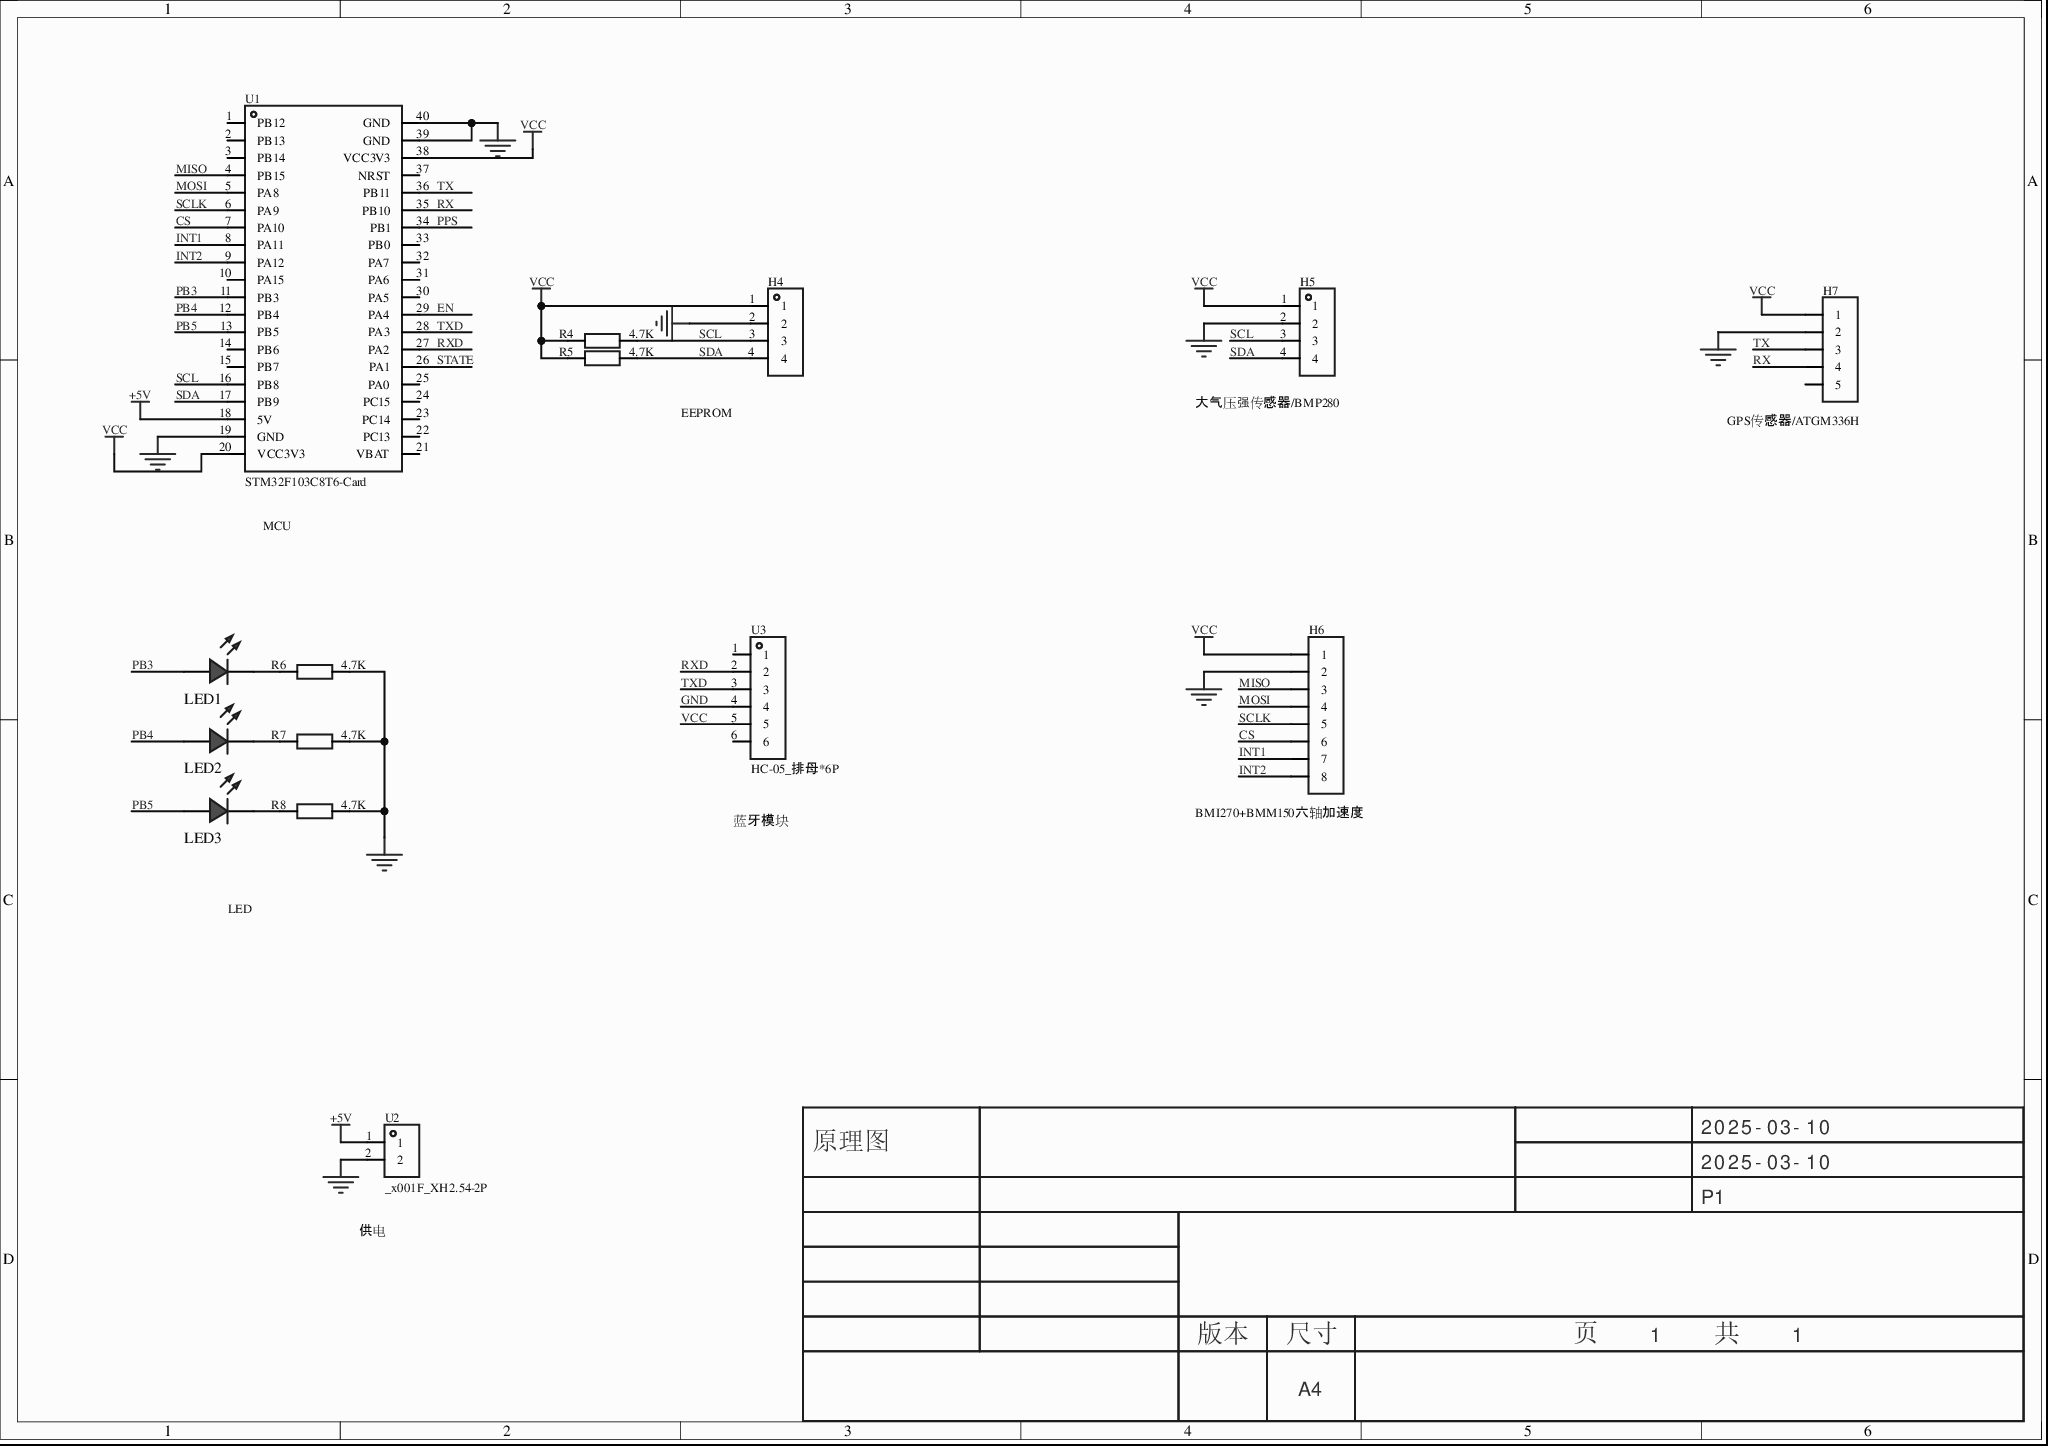
[diagram p0: MISC51830-3.schdoc]
# Altium project MISC51830-2.PrjPcb
1 sheet, 15 parts. Net scope: global (net labels, ports and power ports of the same name join across sheets).
Board file: MISC51830.pcbdoc

## Sheet MISC51830-3.schdoc
size 297 x 209 mm; Version: V1.0; @Project Name: MISC51830; @Page Count: 1; @Update Date: 2025-03-10; @Create Date: 2025-03-10; @Schematic Name: MISC51830; @Page No: 1; @Create Time: 12:29:11; @Update Time: 12:29:16; @Board Name: MISC51830

### Parts
H4  (no value)  [HDR-TH_4P-P2.54-V-F]
H5  (no value)  [HDR-TH_4P-P2.54-V-F]
H6  (no value)  [HDR-TH_8P-P2.54-V-F-1]
H7  (no value)  [HDR-TH_5P-P2.54-V-F]
LED1  (no value)  [LED_0805]
LED2  (no value)  [LED_0805]
LED3  (no value)  [LED_0805]
R4  4.7K  [R0805]
R5  4.7K  [R0805]
R6  4.7K  [R0805]
R7  4.7K  [R0805]
R8  4.7K  [R0805]
U1  STM32F103C8T6-Card  [CONN-TH_L53.3-W22.9_STM32F103C8T6-CARD]
U2  _x001F_XH2.54-2P  [CONN-TH_2P-P2.54-V]
U3  HC-05_排母*6P  [HDR-TH_6P-P2.50-V-F-R1-C6]

### Nets
+5V: U1.18(5V) U2.1
GND: H4.2 H5.2 H6.2 H7.2 R6.2 R7.2 R8.2 U1.19(GND) U1.39(GND) U1.40(GND) U2.2 U3.4
VCC: H4.1 H5.1 H6.1 H7.1 R4.1 R5.1 U1.20(VCC3V3) U1.38(VCC3V3) U3.5
CS: H6.6 U1.7(PA10)
EN: U1.29(PA4)
INT1: H6.7 U1.8(PA11)
INT2: H6.8 U1.9(PA12)
MISO: H6.3 U1.4(PB15)
MOSI: H6.4 U1.5(PA8)
PB3: LED1.2(A) U1.11(PB3)
PB4: LED2.2(A) U1.12(PB4)
PB5: LED3.2(A) U1.13(PB5)
PPS: U1.34(PB1)
RX: H7.4 U1.35(PB10)
RXD: U1.27(PA2) U3.2
SCL: H4.3 H5.3 R4.2 U1.16(PB8)
SCLK: H6.5 U1.6(PA9)
SDA: H4.4 H5.4 R5.2 U1.17(PB9)
STATE: U1.26(PA1)
TX: H7.3 U1.36(PB11)
TXD: U1.28(PA3) U3.3
NetLED1_1: LED1.1(C) R6.1
NetLED2_1: LED2.1(C) R7.1
NetLED3_1: LED3.1(C) R8.1

Not connected (* = marked no-connect by the designer): H7 5*; U1 1(PB12) 2(PB13) 3(PB14) 10(PA15) 14(PB6) 15(PB7) 21(VBAT) 22(PC13) 23(PC14) 24(PC15) 25(PA0) 30(PA5) 31(PA6) 32(PA7) 33(PB0) 37(NRST); U3 1* 6*

### Notes on the sheet
- EEPROM
- (near H5) 大气压强传感器/BMP280
- (near H7) GPS传感器/ATGM336H
- (near U1) MCU
- 蓝牙模块
- (near H6) BMI270+BMM150六轴加速度
- LED
- (near U2) 供电
- 2025-03-10
- 原理图
- P1
- 版本
- 尺寸
- A4
- 页    1    共    1

### Library data of the parts
H4 H5 = HDR-F_2.54_1x4P: Symbol: 2.54-1*4P母; ConvertToPcb: yes; ModelId: d187812051054f85879fcaa51a310d8e; ModelTransform: 419.6842,98.464,0,0,0,0,0,0,-118.11; Device: HDR-F_2.54_1x4P; AddInBom: yes; SupplierPart: C2718488; Supplier Footprint: 插件; FootprintName: HDR-TH_4P-P2.54-V-F; ModelName: HDR-TH_4P-P2.54-V-F
H6 = HDR-F_2.54_1x8P: Symbol: Header-Female-2.54_1x8; AddInBom: yes; ModelId: 0f7e4d9227ef4fa08d5469c22cc70cdb; ModelName: HDR-F-2.54_1x8; ModelTransform: 799.99844,100,0,0,0,0,0,0,-118.11; Device: HDR-F_2.54_1x8P; ConvertToPcb: yes; FootprintName: HDR-TH_8P-P2.54-V-F-1; SupplierPart: C27438; Supplier Footprint: 插件
H7 = HDR-F_2.54_1x5P: Symbol: Header-Female-2.54_1x5; ConvertToPcb: yes; ModelId: f49cb6116a3d45e5a64915bf3e00773f; ModelTransform: 519.684,98.464,0,0,0,0,0,0,-124.016; Device: HDR-F_2.54_1x5P; AddInBom: yes; SupplierPart: C50950; Supplier Footprint: 插件; FootprintName: HDR-TH_5P-P2.54-V-F; ModelName: HDR-TH_5P-P2.54-V-F
LED1-LED3 = LED_0805-R: Symbol: LED_R; Convert to PCB: yes; 3D Model: 33fb9fca58e84f37a403ebeef4c28b77; 3D Model Transform: 78.7,49.1,39.3,0,0,0,0,0,0; ModelName: LED-0805_R; Device: LED_0805-R; Add into BOM: yes; Supplier Footprint: 0805; FootprintName: LED_0805
R4-R8 = Res_0805: ConvertToPcb: yes; SymbolName: 电阻; ModelId: 37a81e68749a4138bd2dfa6897b24b85; ModelName: R0805_L2.0-W1.3-H0.6; ModelTransform: 78.74,51.181,0,0,0,0,0,-0.0005,0; Value: 4.7K; Device: Res_0805; AddInBom: yes; Supplier Footprint: 0805; FootprintName: R0805
U1 = STM32F103C8T6-Card: AddInBom: yes; Symbol: STM32F103C8T6-CARD; Device: STM32F103C8T6-Card; LCSC Part Name: STM32F103C8T6-Card; SupplierPart: C9900077949; ManufacturerPart: STM32F103C8T6-Card; Supplier Footprint: 插件; Supplier: LCSC; ConvertToPcb: yes; FootprintName: CONN-TH_L53.3-W22.9_STM32F103C8T6-CARD
U2 = _x001F_XH2.54-2P: AddInBom: yes; ModelId: 4b619f877c224111ac90f050b36c3583; ModelTransform: 295.275,224.409,0,180,0,0,0,17.717,-118.11; Symbol: _X001F_XH2.54-2P; Device: _x001F_XH2.54-2P; LCSC Part Name: _x001F_XH2.54-2P; SupplierPart: C9900016027; ManufacturerPart: _x001F_XH2.54-2P; Supplier Footprint: XH2.54-2P直插; JLCPCB Part Class: 扩展库; Supplier: LCSC; ConvertToPcb: yes; FootprintName: CONN-TH_2P-P2.54-V; ModelName: CONN-TH_2P-P2.54-V
U3 = HC-05_排母*6P: Symbol: HC-05-*6P; AddInBom: yes; ModelId: 6ff75fbc712a4e2f97a41b366360483c; ModelTransform: 590.55,98.425,0,0,0,0,0,0,-118.11; Device: HC-05_排母*6P; LCSC Part Name: HC-05_排母*6P; SupplierPart: C9900003093; ManufacturerPart: HC-05_排母*6P; Supplier Footprint: TH-6_2.5X15.6X2.54P; JLCPCB Part Class: 扩展库; Supplier: LCSC; ConvertToPcb: yes; FootprintName: HDR-TH_6P-P2.50-V-F-R1-C6; ModelName: HDR-TH_6P-P2.50-V-F-R1-C6